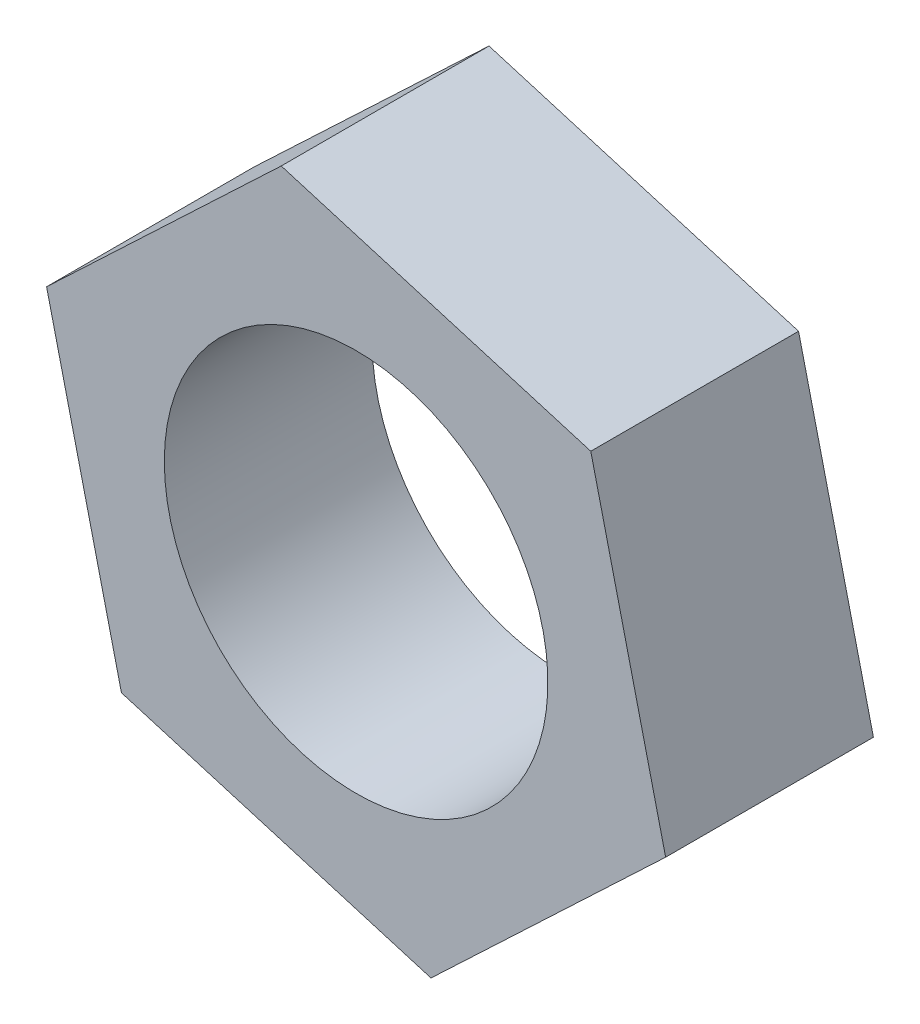
from build123d import *

# Parameters (mm, degrees)
SKETCH1_R           = 24
BOSS_EXTRUDE1_DEPTH = 26


with BuildPart() as part:
    # Sketch1 → Boss-Extrude1 (new body)
    with BuildSketch(Plane.XY):
        Polygon((38.730527716, -11.544676531), (29.363247012, 27.769282638), (-9.367280704, 39.313959169), (-38.730527716, 11.544676531), (-29.363247012, -27.769282638), (9.367280704, -39.313959169), align=None)
        with Locations(Location((0, 0, 0), (0, 0, 180))):
            Circle(SKETCH1_R, mode=Mode.SUBTRACT)
    extrude(amount=BOSS_EXTRUDE1_DEPTH)


solid = part.part
